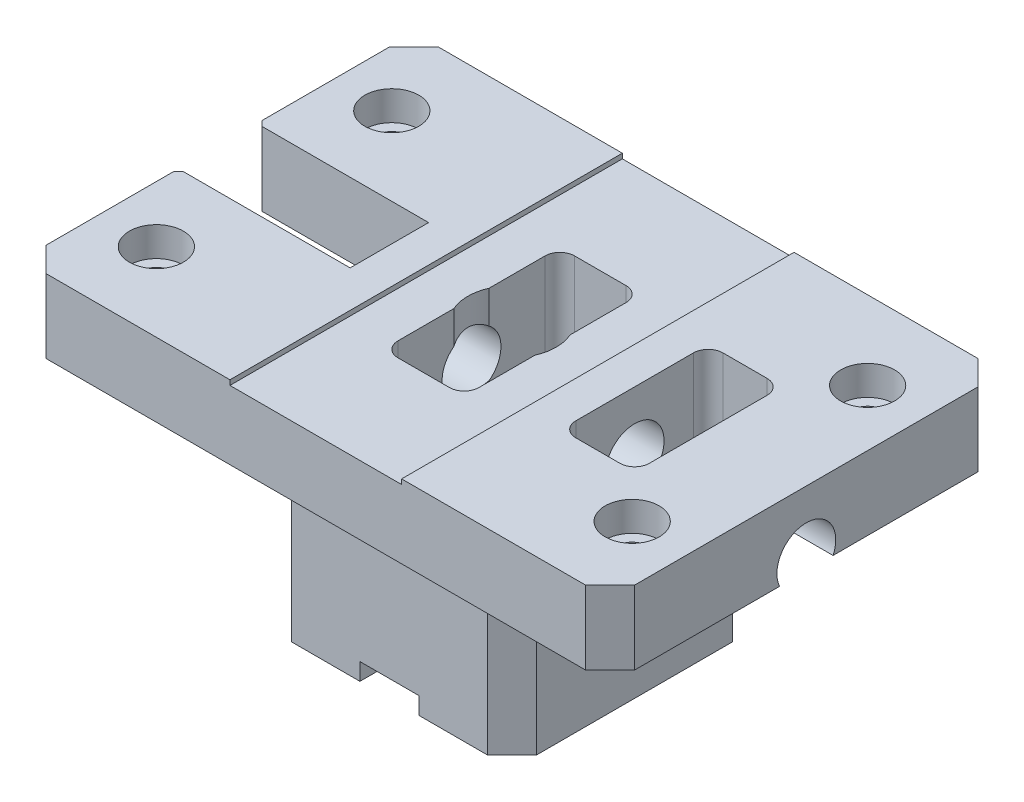
from build123d import *

# Parameters (mm, degrees)
SKETCH1_W                                            = 120
SKETCH1_H                                            = 80
BOSS_EXTRUDE1_DEPTH                                  = 15
SKETCH2_W                                            = 50
SKETCH2_H                                            = 50
BOSS_EXTRUDE2_DEPTH                                  = 40
CUT_EXTRUDE2_DEPTH                                   = 33
SKETCH5_W                                            = 16
SKETCH5_H                                            = 41.240104646
CUT_EXTRUDE3_DEPTH                                   = 35
SKETCH6_R                                            = 6
CUT_EXTRUDE4_DEPTH                                   = 103.102889283
CBORE_FOR_M6_HEX_SOCKET_HEAD_CAP_SCREW1_D            = 6.6
CBORE_FOR_M6_HEX_SOCKET_HEAD_CAP_SCREW1_CBORE_D      = 11
CBORE_FOR_M6_HEX_SOCKET_HEAD_CAP_SCREW1_CBORE_DEPTH  = 6
SKETCH11_W                                           = 12
SKETCH11_H                                           = 60
CUT_EXTRUDE5_DEPTH                                   = 3.5
CUT_EXTRUDE7_DEPTH                                   = 91.691785736
CHAMFER1_SIZE                                        = 5
CHAMFER2_SIZE                                        = 1
SKETCH14_W                                           = 35
SKETCH14_H                                           = 80
CUT_EXTRUDE8_DEPTH                                   = 1
CBORE_FOR_M10_HEX_SOCKET_HEAD_CAP_SCREW1_D           = 11
CBORE_FOR_M10_HEX_SOCKET_HEAD_CAP_SCREW1_CBORE_D     = 18
CBORE_FOR_M10_HEX_SOCKET_HEAD_CAP_SCREW1_CBORE_DEPTH = 42


with BuildPart() as part:
    # Sketch1 → Boss-Extrude1 (new body)
    with BuildSketch(Plane(origin=(0, 0, 0), x_dir=(1, 0, 0), z_dir=(0, 1, 0))):
        Rectangle(SKETCH1_W, SKETCH1_H)
    extrude(amount=BOSS_EXTRUDE1_DEPTH)

    # Sketch2 → Boss-Extrude2 (add)
    with BuildSketch(Plane.XZ):
        Rectangle(SKETCH2_W, SKETCH2_H)
    extrude(amount=BOSS_EXTRUDE2_DEPTH)

    # Sketch4 → Cut-Extrude2 (cut)
    with BuildSketch(Plane(origin=(0, 15, 0), x_dir=(1, 0, 0), z_dir=(0, 1, 0))):
        with BuildLine():
            Line((-5.25, 18), (5.25, 18))
            ThreePointArc((5.25, 18), (7.371320344, 17.121320344), (8.25, 15))
            Line((8.25, 15), (8.25, -15))
            ThreePointArc((8.25, -15), (7.371320344, -17.121320344), (5.25, -18))
            Line((5.25, -18), (-5.25, -18))
            ThreePointArc((-5.25, -18), (-7.371320344, -17.121320344), (-8.25, -15))
            Line((-8.25, -15), (-8.25, 15))
            ThreePointArc((-8.25, 15), (-7.371320344, 17.121320344), (-5.25, 18))
        make_face()
    extrude(amount=-CUT_EXTRUDE2_DEPTH, mode=Mode.SUBTRACT)

    # Sketch5 → Cut-Extrude3 (cut)
    with BuildSketch(Plane.ZY.offset(60)):
        Rectangle(SKETCH5_W, SKETCH5_H)
    extrude(amount=-CUT_EXTRUDE3_DEPTH, mode=Mode.SUBTRACT)

    # Sketch6 → Cut-Extrude4 (cut, through all)
    with BuildSketch(Plane.ZY.offset(25)):
        with Locations(Location((0, 2.5, 0), (0, 0, 335.375681648))):
            Circle(SKETCH6_R)
    extrude(amount=-CUT_EXTRUDE4_DEPTH, mode=Mode.SUBTRACT)

    # CBORE for M6 Hex Socket Head Cap Screw1 (through all)
    with Locations(Plane(origin=(0, 15, 0), x_dir=(-1, 0, 0), z_dir=(0, 1, 0))):
        with Locations((48.5, 24), (-48.5, 24), (-48.5, -24), (48.5, -24)):
            CounterBoreHole(CBORE_FOR_M6_HEX_SOCKET_HEAD_CAP_SCREW1_D / 2, CBORE_FOR_M6_HEX_SOCKET_HEAD_CAP_SCREW1_CBORE_D / 2, CBORE_FOR_M6_HEX_SOCKET_HEAD_CAP_SCREW1_CBORE_DEPTH)

    # Sketch11 → Cut-Extrude5 (cut)
    with BuildSketch(Plane.XZ.offset(40)):
        Rectangle(SKETCH11_W, SKETCH11_H)
    extrude(amount=-CUT_EXTRUDE5_DEPTH, mode=Mode.SUBTRACT)

    # Sketch13 → Cut-Extrude7 (cut, through all)
    with BuildSketch(Plane(origin=(0, 15, 0), x_dir=(1, 0, 0), z_dir=(0, 1, 0))):
        with BuildLine():
            Line((28, 15), (37, 15))
            ThreePointArc((37, 15), (39.121320344, 14.121320344), (40, 12))
            Line((40, 12), (40, -12))
            ThreePointArc((40, -12), (39.121320344, -14.121320344), (37, -15))
            Line((37, -15), (28, -15))
            ThreePointArc((28, -15), (25.878679656, -14.121320344), (25, -12))
            Line((25, -12), (25, 12))
            ThreePointArc((25, 12), (25.878679656, 14.121320344), (28, 15))
        make_face()
    extrude(amount=-CUT_EXTRUDE7_DEPTH, mode=Mode.SUBTRACT)

    # Chamfer1
    chamfer1_edges = [part.edges().sort_by_distance(p)[0] for p in [
        (25, -20, -25),
        (25, -20, 25),
        (-25, -20, 25),
        (-25, -20, -25),
        (60, 7.5, 40),
        (-60, 7.5, 40),
        (-60, 7.5, -40),
        (60, 7.5, -40),
    ]]
    chamfer(chamfer1_edges, length=CHAMFER1_SIZE)

    # Chamfer2
    chamfer2_edges = [part.edges().sort_by_distance(p)[0] for p in [
        (-60, 7.5, -8),
        (-60, 7.5, 8),
    ]]
    chamfer(chamfer2_edges, length=CHAMFER2_SIZE)

    # Sketch14 → Cut-Extrude8 (cut)
    with BuildSketch(Plane(origin=(0, 15, 0), x_dir=(1, 0, 0), z_dir=(0, 1, 0))):
        Rectangle(SKETCH14_W, SKETCH14_H)
    extrude(amount=-CUT_EXTRUDE8_DEPTH, mode=Mode.SUBTRACT)

    # CBORE for M10 Hex Socket Head Cap Screw1 (through all)
    with Locations(Plane(origin=(-12.636834377, 14, 0.883421015), x_dir=(-1, 0, 0), z_dir=(0, 1, 0))):
        with Locations((-12.636834377, -0.883421015)):
            CounterBoreHole(CBORE_FOR_M10_HEX_SOCKET_HEAD_CAP_SCREW1_D / 2, CBORE_FOR_M10_HEX_SOCKET_HEAD_CAP_SCREW1_CBORE_D / 2, CBORE_FOR_M10_HEX_SOCKET_HEAD_CAP_SCREW1_CBORE_DEPTH)


solid = part.part
